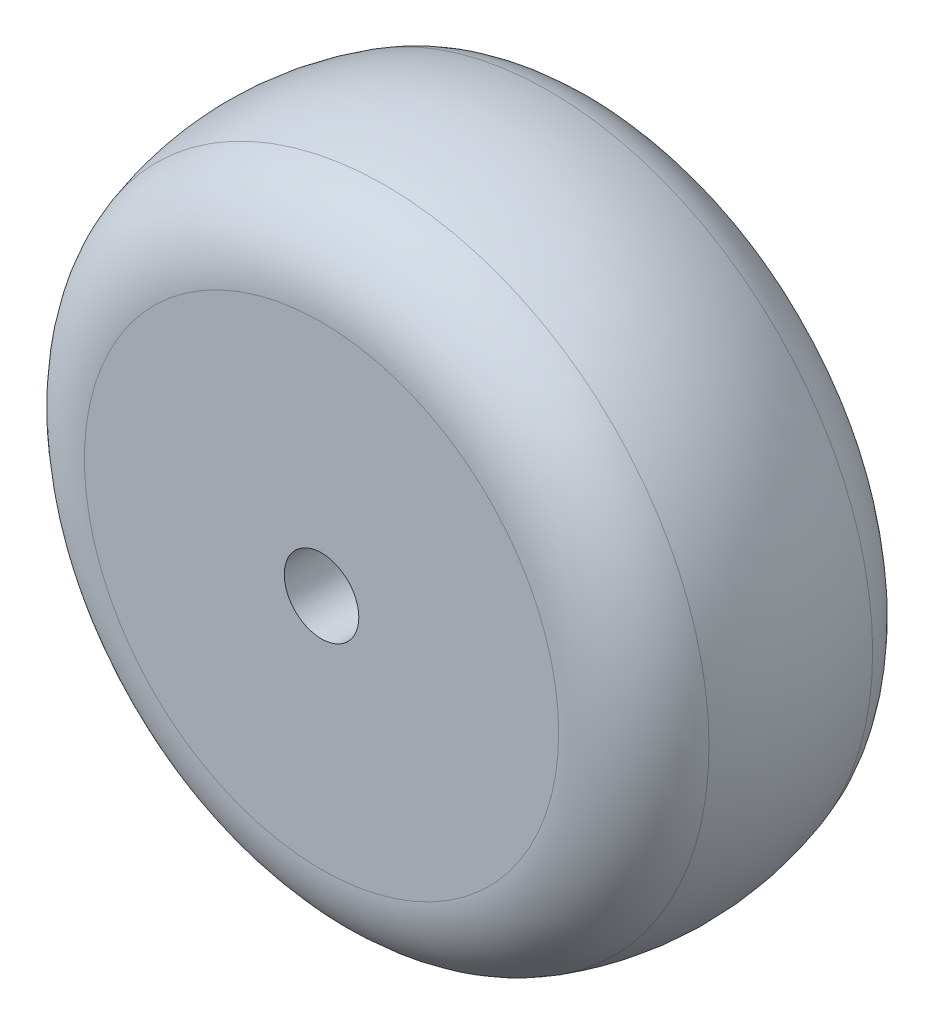
SolidWorks part; units mm, degrees
ref_plane "前视基准面" through (0, 0, 0) normal (0, 0, 1) x (1, 0, 0)
ref_plane "上视基准面" through (0, 0, 0) normal (0, 1, 0) x (1, 0, 0)
ref_plane "右视基准面" through (0, 0, 0) normal (1, 0, 0) x (0, 0, -1)
sketch "草图1" plane through (0, 0, 0) normal (0, 1, 0) x (1, 0, 0)
  line L0 (0, 0) -> (0, 42.7086) construction
  line L1 (0, 0) -> (27.9184, 0) construction
  line L2 (4.1, 16) -> (32.3772, 16)
  line L3 (4.1, 16) -> (4.1, -16)
  line L4 (4.1, -16) -> (32.3772, -16)
  arc A0 (32.3772, 16) -> (32.3772, -16) centre (7, 0) cw
  dimension "D1" = 74
  dimension "D3" = 30
  dimension "D2" = 32
  dimension "D4" = 8.2
revolve "旋转1" add sketch "草图1" angle 360 about L0
fillet "圆角1" radius 10 2 edges at (32.3772, 0, -16) (32.3772, 0, 16)
